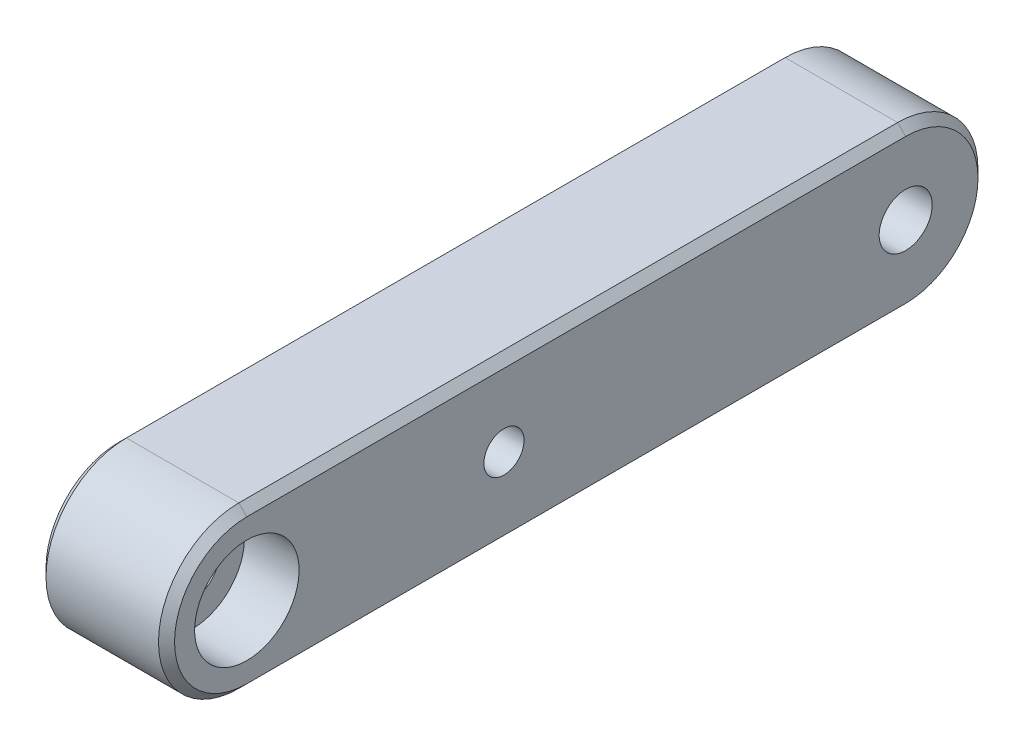
SolidWorks part; units mm, degrees
material "6061"
ref_plane "前视基准面" through (0, 0, 0) normal (0, 0, 1) x (1, 0, 0)
ref_plane "上视基准面" through (0, 0, 0) normal (0, 1, 0) x (1, 0, 0)
ref_plane "右视基准面" through (0, 0, 0) normal (1, 0, 0) x (0, 0, -1)
sketch "草图1" plane through (0, 0, 0) normal (1, 0, 0) x (0, 0, -1)
  line L0 (20.5, 0) -> (-20.5, 0) construction
  line L1 (20.5, -5) -> (-20.5, -5)
  line L2 (20.5, 5) -> (-20.5, 5)
  arc A0 (20.5, -5) -> (20.5, 5) centre (20.5, 0) ccw
  arc A1 (-20.5, 5) -> (-20.5, -5) centre (-20.5, 0) ccw
  point P2 (0, 0)
  dimension "D2" = 5
  dimension "D1" = 41
extrude "凸台-拉伸1" add sketch "草图1" along normal mid plane 8
hole_wizard "打孔尺寸(%根据)内六角圆柱头螺钉的类型1" positions "草图3" profile "草图2" counterbore size "M3" standard "GB" end condition through all
sketch "草图3" plane through (4, 0, 0) normal (1, 0, 0) x (0, 0, -1)
  point P0 (-20.5, 0)
sketch "草图2" plane through (4, 0, 20.5) normal (0, 1, 0) x (0, 0, -1)
  line L0 (0, 0) -> (0, 8)
  line L1 (0, 8) -> (1.7, 8)
  line L3 (1.7, 8) -> (1.7, 3.4)
  line L4 (1.7, 3.4) -> (3.25, 3.4)
  line L5 (3.25, 3.4) -> (3.25, 0)
  line L7 (3.25, 0) -> (0, 0)
  line L11 (0, -6.35) -> (0, 107.95) construction
  dimension "通孔孔直径" = 3.4
  dimension "通孔孔深度" = 8
  dimension "柱形沉头孔直径" = 6.5
  dimension "柱形沉头孔深度" = 3.4
hole_wizard "M3 螺纹孔1" positions "草图5" profile "草图4" tap size "M3" standard "GB" end condition through all
sketch "草图5" plane through (4, 0, 0) normal (1, 0, 0) x (0, 0, -1)
  circle A0 centre (-20.5, 0) radius 1.7 construction
  point P0 (-4.5, 0)
  dimension "D1" = 16
sketch "草图4" plane through (4, 0, 4.5) normal (0, 1, 0) x (0, 0, -1)
  line L0 (0, 0) -> (0, 8)
  line L1 (0, 8) -> (1.25, 8)
  line L2 (1.25, 8) -> (1.25, 0)
  line L5 (1.25, 0) -> (0, 0)
  line L11 (0, -6.35) -> (0, 107.95) construction
  dimension "通孔螺纹孔钻头直径" = 2.5
  dimension "通孔螺纹孔钻头深度" = 8
cosmetic thread "孔螺蚊线1" parameters "D2"=3
hole_wizard "M4 螺纹孔1" positions "草图7" profile "草图6" tap size "M4" standard "GB" end condition through all
sketch "草图7" plane through (4, 0, 0) normal (1, 0, 0) x (0, 0, -1)
  point P0 (20.5, 0)
sketch "草图6" plane through (4, 0, -20.5) normal (0, 1, 0) x (0, 0, -1)
  line L0 (0, 0) -> (0, 8)
  line L1 (0, 8) -> (1.65, 8)
  line L2 (1.65, 8) -> (1.65, 0)
  line L5 (1.65, 0) -> (0, 0)
  line L11 (0, -6.35) -> (0, 107.95) construction
  dimension "通孔螺纹孔钻头直径" = 3.3
  dimension "通孔螺纹孔钻头深度" = 8
cosmetic thread "孔螺蚊线2"
chamfer "倒角1" distance 0.5 angle 45 8 edges at (-4, 5, 0) (-4, 0, 25.5) (-4, 0, -25.5) (-4, -5, 0) (4, 5, 0) (4, 0, 25.5) (4, 0, -25.5) (4, -5, 0)
